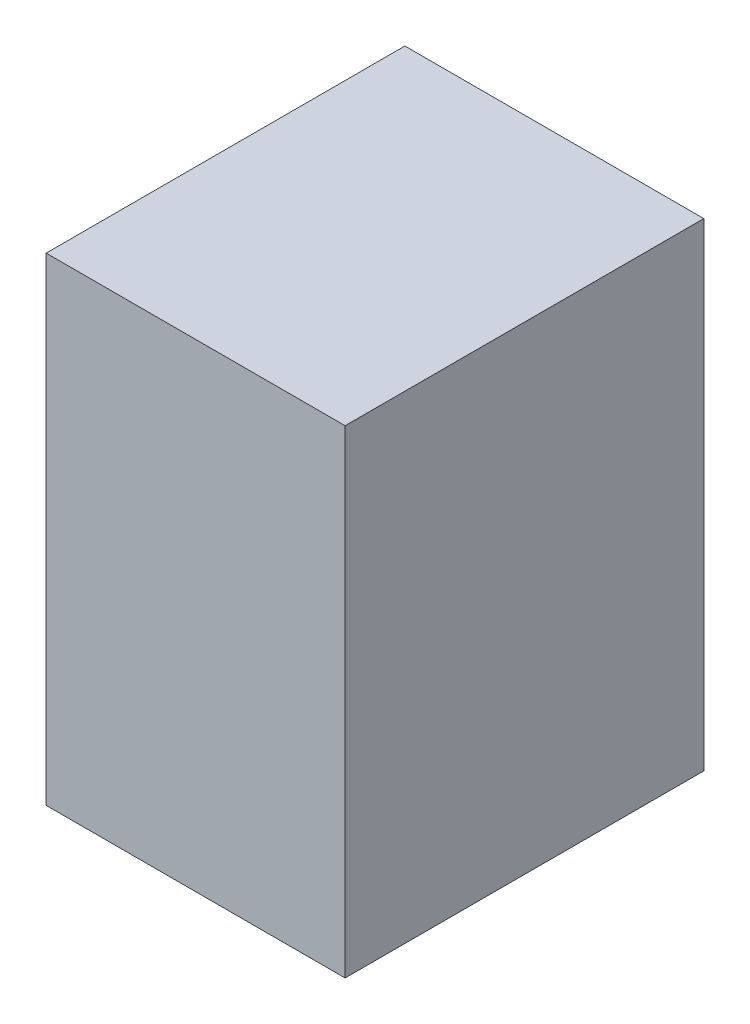
SolidWorks part; units mm, degrees
ref_plane "Front Plane" through (0, 0, 0) normal (0, 0, 1) x (1, 0, 0)
ref_plane "Top Plane" through (0, 0, 0) normal (0, 1, 0) x (1, 0, 0)
ref_plane "Right Plane" through (0, 0, 0) normal (1, 0, 0) x (0, 0, -1)
sketch "Sketch1" plane through (0, 0, 0) normal (0, 0, 1) x (1, 0, 0)
  line L1 (-125, 200) -> (125, 200)
  line L2 (-125, 200) -> (-125, -200)
  line L3 (-125, -200) -> (125, -200)
  line L4 (125, 200) -> (125, -200)
  line L5 (-125, 200) -> (125, -200) construction
  line L6 (-125, -200) -> (125, 200) construction
  point P0 (0, 0)
  dimension "D1" = 250
  dimension "D2" = 400
extrude "Boss-Extrude1" add sketch "Sketch1" along normal blind 300
